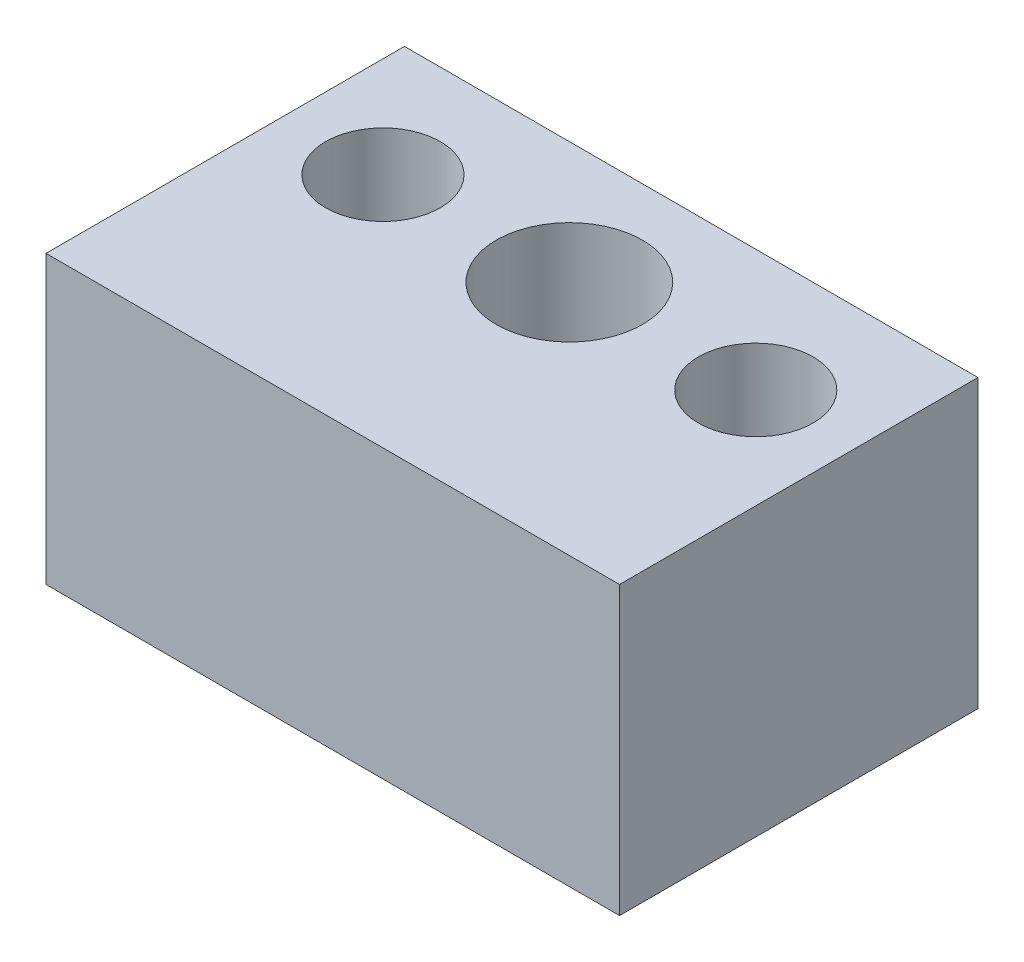
SolidWorks part; units mm, degrees
ref_plane "前视基准面" through (0, 0, 0) normal (0, 0, 1) x (1, 0, 0)
ref_plane "上视基准面" through (0, 0, 0) normal (0, 1, 0) x (1, 0, 0)
ref_plane "右视基准面" through (0, 0, 0) normal (1, 0, 0) x (0, 0, -1)
sketch "草图1" plane through (0, 0, 0) normal (0, 0, 1) x (1, 0, 0)
  line L1 (-20, -10) -> (20, -10)
  line L2 (-20, -10) -> (-20, 10)
  line L3 (-20, 10) -> (20, 10)
  line L4 (20, -10) -> (20, 10)
  line L5 (-20, -10) -> (20, 10) construction
  line L6 (-20, 10) -> (20, -10) construction
  point P0 (0, 0)
  dimension "D1" = 20
  dimension "D2" = 40
extrude "凸台-拉伸1" add sketch "草图1" along normal mid plane 17
sketch "草图2" plane through (0, 10, 0) normal (0, 1, 0) x (1, 0, 0)
  line L0 (-20, -8.5) -> (-20, 8.5) construction
  line L1 (20, -8.5) -> (20, 8.5) construction
  circle A0 centre (-13, 0) radius 4
  circle A1 centre (13, 0) radius 4
extrude "切除-拉伸1" cut sketch "草图2" against normal up to next
sketch "草图3" plane through (0, -10, 0) normal (0, -1, 0) x (1, 0, 0)
  circle A0 centre (0, 0) radius 4
  dimension "D1" = 8
extrude "切除-拉伸2" cut sketch "草图3" against normal up to next
sketch "草图4" plane through (0, 0, 8.5) normal (0, 0, 1) x (1, 0, 0)
  line L0 (20, -10) -> (20, 10) construction
  line L2 (-20, 10) -> (-20, -10) construction
  circle A0 centre (14.5, 0) radius 2.75
  circle A1 centre (-14.5, 0) radius 2.75
  dimension "D3" = 5.5
  dimension "D1" = 5.5
  dimension "D2" = 5.5
extrude "切除-拉伸3" [suppressed] cut sketch "草图4" against normal up to next
sketch "草图5" plane through (0, 0, 8.5) normal (0, 0, 1) x (1, 0, 0)
  line L0 (-20, 10) -> (-20, -10) construction
  line L5 (20, -10) -> (-20, -10)
  line L6 (20, -10) -> (20, 15)
  line L7 (20, 15) -> (-20, 15)
  line L8 (-20, -10) -> (-20, 15)
  dimension "D1" = 25
extrude "凸台-拉伸2" [suppressed] add sketch "草图5" along normal blind 6
sketch "草图6" plane through (0, 0, 8.5) normal (0, 0, 1) x (1, 0, 0)
  line L1 (-20, -10) -> (20, -10)
  line L2 (-20, -10) -> (-20, 10)
  line L3 (-20, 10) -> (20, 10)
  line L4 (20, -10) -> (20, 10)
extrude "凸台-拉伸3" add sketch "草图6" along normal blind 8
hole_wizard "M12 螺纹孔1" positions "3D草图1" profile "草图7" tap size "M12" standard "GB" end condition up to next
sketch3d "3D草图1"
  circle A0 centre (0, 10, 0) radius 4 construction
  point P8 (0, 10, 0)
  point P12 (0, 14, 0)
sketch "草图7" plane through (0, 10, 0) normal (1, 0, 0) x (0, 0, 1)
  line L0 (0, 0) -> (0, 20)
  line L1 (0, 20) -> (5.1, 20)
  line L2 (5.1, 20) -> (5.1, 0)
  line L5 (5.1, 0) -> (0, 0)
  line L11 (0, -6.35) -> (0, 107.95) construction
  dimension "通孔螺纹孔钻头直径" = 10.2
  dimension "通孔螺纹孔钻头深度" = 20
cosmetic thread "孔螺蚊线1" parameters "D2"=12
equation "\"D1@草图2\"=\"D2@草图2\""
